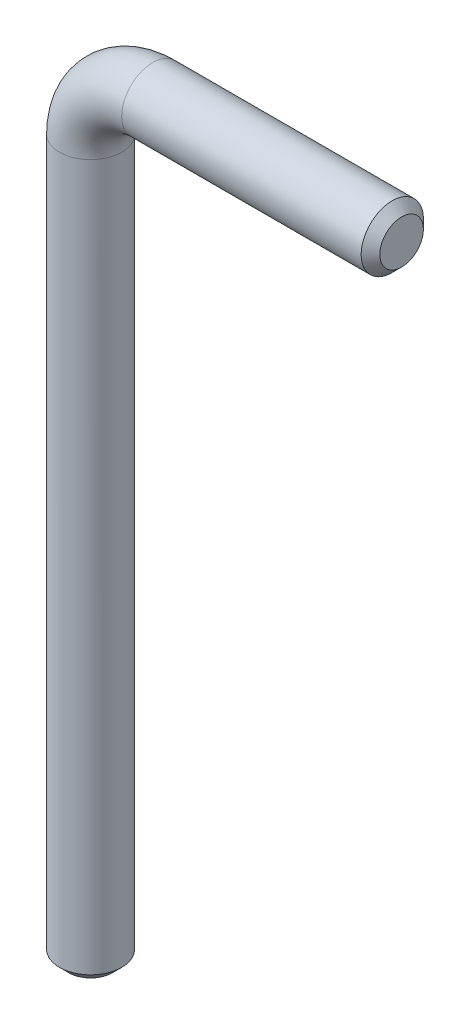
from build123d import *

# Parameters (mm, degrees)
SWEEP_1_PROFILE_R = 10
CHAMFER_1_SIZE    = 3
CHAMFER_2_SIZE    = 3


with BuildPart() as part:
    # 扫描1: sweep along a path in 草图1
    with BuildLine(Plane.XY) as sweep_1_path:
        Line((0, -250), (0, -20))
        ThreePointArc((0, -20), (5.857864376, -5.857864376), (20, 0))
        Line((20, 0), (100, 0))
    # 扫描1 profile (on start of the path) → 扫描1 (sweep)
    with BuildSketch(Plane(origin=(0, -250, 0), x_dir=(1, 0, 0), z_dir=(0, 1, 0))):
        Circle(SWEEP_1_PROFILE_R)
    sweep(path=sweep_1_path.line)

    # 倒角1
    chamfer_1_edges = [part.edges().sort_by_distance(p)[0] for p in [
        (-10, -250, 0),
    ]]
    chamfer(chamfer_1_edges, length=CHAMFER_1_SIZE)

    # 倒角2
    chamfer_2_edges = [part.edges().sort_by_distance(p)[0] for p in [
        (100, 10, 0),
    ]]
    chamfer(chamfer_2_edges, length=CHAMFER_2_SIZE)


solid = part.part
